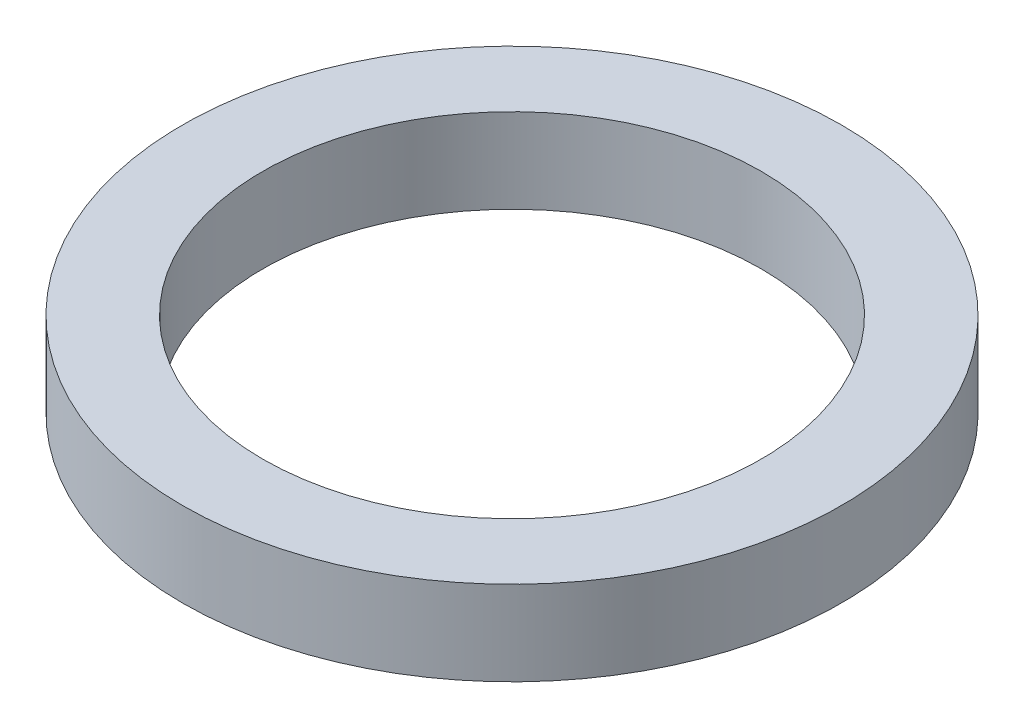
from build123d import *

# Parameters (mm, degrees)
SKETCH1_R           = 7.8
SKETCH1_R_2         = 5.9
BOSS_EXTRUDE1_DEPTH = 2


with BuildPart() as part:
    # Sketch1 → Boss-Extrude1 (new body)
    with BuildSketch(Plane(origin=(0, 0, 0), x_dir=(1, 0, 0), z_dir=(0, 1, 0))):
        with Locations(Location((0, 0, 0), (0, 0, 270))):
            Circle(SKETCH1_R)
        with Locations(Location((0, 0, 0), (0, 0, 270))):
            Circle(SKETCH1_R_2, mode=Mode.SUBTRACT)
    extrude(amount=BOSS_EXTRUDE1_DEPTH)


solid = part.part
